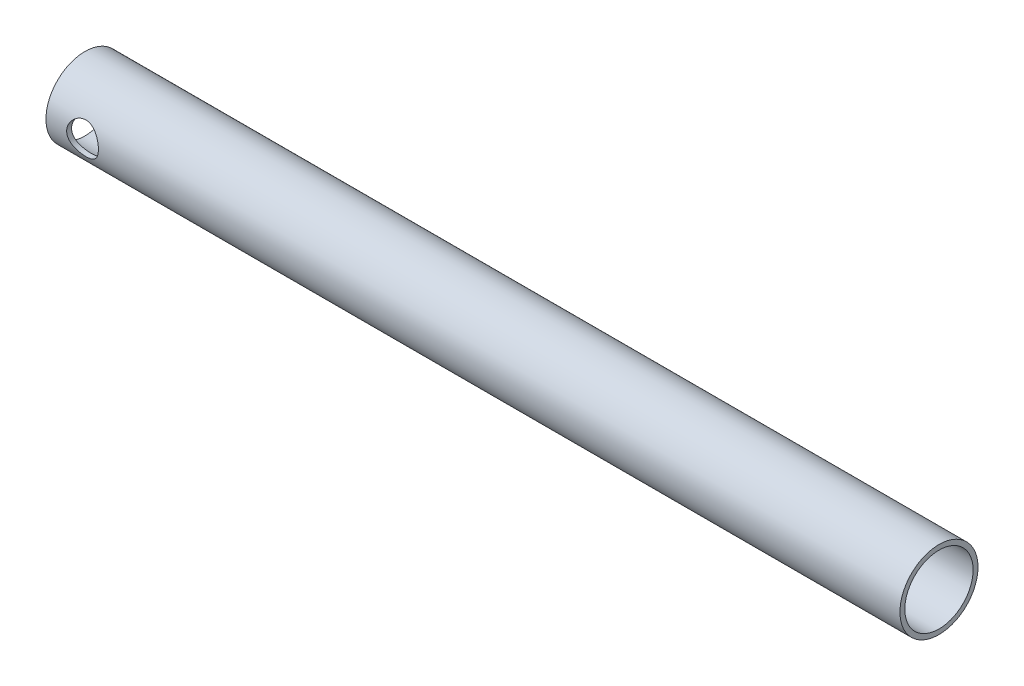
from build123d import *

# Parameters (mm, degrees)
SWEEP_1_PROFILE_R        = 16
SWEEP_1_PROFILE_R_2      = 14
CUT_EXTRUDE_1_DEPTH      = 177.456793578
CUT_EXTRUDE_1_DEPTH_BACK = 177.456793578
SKETCH_26_R              = 6.5


with BuildPart() as part:
    # 扫描-薄件1: sweep along a path in 草图1
    with BuildLine(Plane.XY) as sweep_1_path:
        Line((-175, 0), (175, 0))
    # 扫描-薄件1 profile (on start of the path) → 扫描-薄件1 (sweep)
    with BuildSketch(Plane(origin=(-175, 0, 0), x_dir=(0, 0, 1), z_dir=(1, 0, 0))):
        Circle(SWEEP_1_PROFILE_R)
        Circle(SWEEP_1_PROFILE_R_2, mode=Mode.SUBTRACT)
    sweep(path=sweep_1_path.line)

    # 草图26 → 切除-拉伸1 (cut, two sides: drawn at the far end of the back side and taken through both)
    with BuildSketch(Plane.XY.offset(-CUT_EXTRUDE_1_DEPTH_BACK)):
        with Locations((-160, 0)):
            Circle(SKETCH_26_R)
    extrude(amount=CUT_EXTRUDE_1_DEPTH + CUT_EXTRUDE_1_DEPTH_BACK, mode=Mode.SUBTRACT)


solid = part.part
